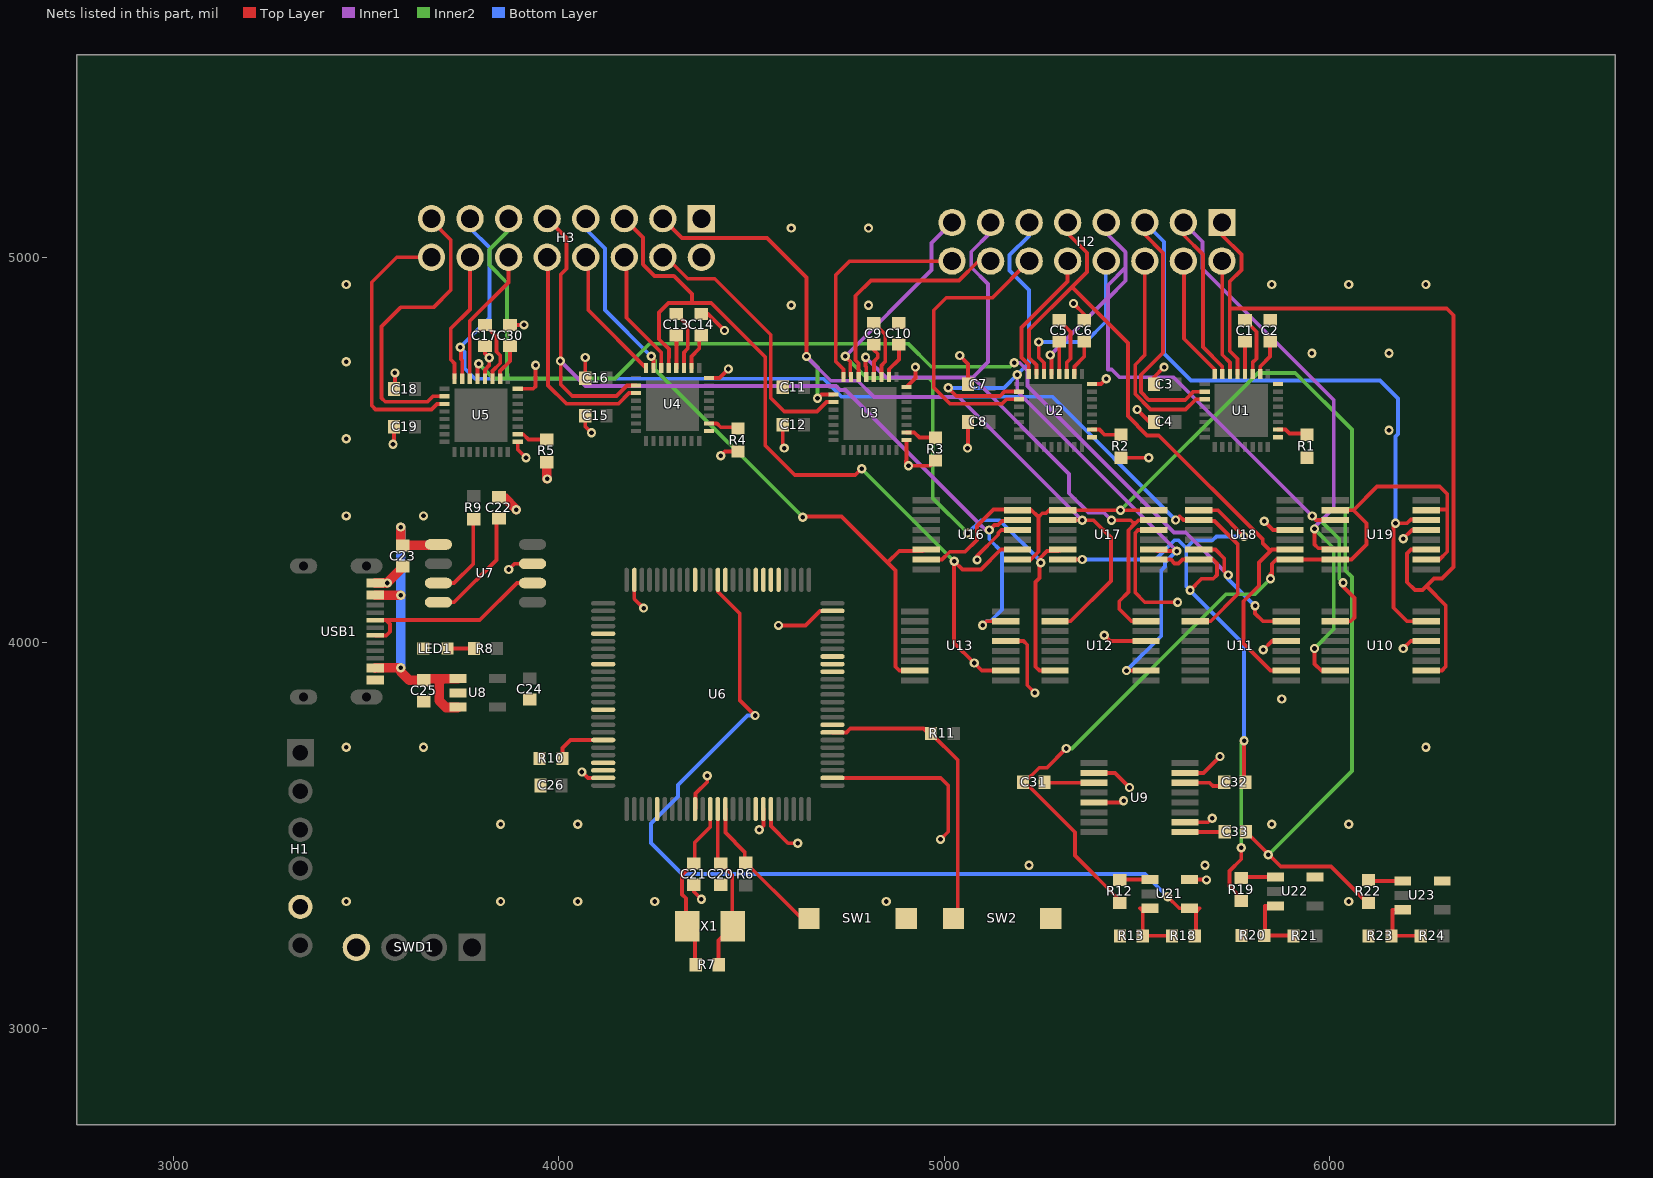
[diagram p0: the nets of this part, all layers, seen from the top]
# Altium PCB MISC49858.pcbdoc (part 2 of 3)
Units mil, origin at the board's own origin, x right, y up, seen from the top; angles counter-clockwise.
Board outline 3990 x 2775 mil, 6 copper layers (Top Layer, Inner1, Inner2, Inner3, Inner4, Bottom Layer), stack 60.565 mil thick; 79 components, 151 nets, 603 pads, 275 vias.

## Via types
v1: diameter 24.02, hole 12, Top Layer to Bottom Layer, 275 vias

## Nets (pads, with @x,y where several pads share a name; then routed paths per layer and width w, separated by ;. In a path a pad name is that pad's centre, name@x,y a point inside that pad or via, vN(x,y) a via of type N, cw(c..) or ccw(c..) an arc to the next point about the centre after c; other vN are vias at no path point) (continued)
$2N132: U7.2 USB1.A7 USB1.B7 | length 550.9
  Top Layer w10: USB1.A7@3524.29,4019.26 3552.56,4019.26 3561.93,4028.63 3561.93,4048.63 3551.93,4058.63 USB1.B7@3524.29,4058.63 3795.2,4058.63 3891.57,4154.99 U7.2@3932,4155
$2N186: C22.1 U7.8 | length 305.9
  Top Layer w10: U7.8@3688,4105 3728.43,4105 3838.43,4214.99 3838.43,4314.99 C22.1@3845,4322.44
$2N192: R9.1 U7.7 | length 227
  Top Layer w10: U7.7@3688,4155 3728.43,4154.99 3778.43,4204.99 3778.43,4314.99 R9.1@3779.66,4320.68
$2N294: LED1.1 R8.1 | length 68.9
  Top Layer w10: LED1.1@3711.47,3985.01 R8.1@3780.34,3985
$2N443: C30.1 U5.26 | length 95.2
  Top Layer w9.92: U5.26@3848.02,4684.78 3848.01,4704.78 3873.59,4730.35 C30.1@3873.59,4769.38
$2N495: R5.2 U5.18 | length 80.8
  Top Layer w9.92: U5.18@3893.59,4540.79 3907.98,4540.79 3921.39,4527.37 R5.2@3968.81,4527.37
$2N1063: C14.1 U4.26 | length 95.2
  Top Layer w9.92: U4.26@4344.43,4712.84 4344.43,4742.84 4364.43,4762.84 4364.43,4791.87 C14.1@4370,4797.44
$2N1115: R4.2 U4.18 | length 80.4
  Top Layer w9.92: U4.18@4390,4568.85 4410,4568.86 4420,4558.86 4460,4558.86 R4.2@4465.22,4555.43
$2N1219: C10.1 U3.26 | length 95.2
  Top Layer w9.92: U3.26@4856.57,4689.46 4856.57,4709.46 4882.14,4735.03 C10.1@4882.14,4774.06
$2N1271: R3.2 U3.18 | length 80.8
  Top Layer w9.92: U3.18@4902.14,4545.47 4922.14,4545.47 4935.56,4532.05 R3.2@4977.36,4532.05
$2N1375: C6.1 U2.26 | length 95.2
  Top Layer w9.92: U2.26@5337.29,4696.84 5337.29,4716.84 5362.87,4742.42 C6.1@5362.87,4781.44
$2N1427: R2.2 U2.18 | length 80.8
  Top Layer w9.92: U2.18@5382.86,4552.85 5402.15,4552.85 5415.57,4539.43 R2.2@5458.08,4539.43
$2N1634: R1.2 U1.18 | length 80.4
  Top Layer w9.92: U1.18@5864.97,4552.85 5884.97,4552.86 5894.97,4542.86 5934.97,4542.86 R1.2@5940.19,4539.43
$2N1686: C2.1 U1.26 | length 95.2
  Top Layer w9.92: U1.26@5819.4,4696.84 5819.4,4716.84 5844.97,4742.42 C2.1@5844.97,4781.44
$2N21184: U6.90
$2N21229: U6.18
$2N21235: U6.34
$2N21247: U6.66
$2N21259: U6.80
$2N21271: U6.84
$2N21286: U6.55
$2N21289: U6.56
$2N21292: U6.57
$2N21295: U6.58
$2N21307: U6.62
$2N21310: U6.97
$2N21317: U6.98
$2N21332: U6.5
$2N21344: U6.41
$2N21348: U6.42
$2N21351: U6.43
$2N24751: R10.1 U6.94 | length 141.3
  Top Layer w10: R10.1@4009.66,3700 4009.66,3726.95 4030.59,3747.88 U6.94@4115.29,3747.88
$2N29551: C32.2 U9.14 | length 109.4
  Top Layer w10: U9.14@5624.33,3636.93 5688.08,3636.93 5696.46,3628.55 5716.46,3628.55 C32.2@5725.93,3638.55
$2N29571: C33.2 U9.9 | length 103.1
  Top Layer w10: U9.9@5624.33,3508.98 5714.83,3508.98 C33.2@5727.44,3510
$2N29592: C31.1 U9.3 | length 129.4
  Top Layer w10: C31.1@5259.37,3638.55 5265.99,3638.55 5267.61,3636.93 U9.3@5388.11,3636.93
$2N29599: R12.2 U21.1 | length 78.6
  Top Layer w10: R12.2@5455,3384.66 5466.88,3386.25 U21.1@5533.53,3386.25
$2N29605: R13.2 R18.1 U21.3 | length 177
  Top Layer w10: U21.3@5533.53,3311.45 5506.88,3311.45 5514.66,3303.67 R13.2@5514.66,3240 R18.1@5590.34,3240
$2N29606: R20.2 R21.1 U22.3 | length 179.7
  Top Layer w10: U22.3@5858.81,3317.6 5832.16,3317.6 5832.16,3247.6 5829.92,3245.36 R20.2@5829.92,3241.02 5899.92,3241.02 R21.1@5905.34,3240
$2N29610: R19.2 U22.1 | length 89.1
  Top Layer w10: R19.2@5770,3389.66 5782.16,3392.4 U22.1@5858.81,3392.4
$2N29613: R23.2 R24.1 U23.3 | length 171
  Top Layer w10: U23.3@6188.81,3307.6 6162.16,3307.6 6162.16,3247.6 6159.66,3245.1 R23.2@6159.66,3240 R24.1@6235.34,3240
$2N29617: R22.2 U23.1 | length 89.8
  Top Layer w10: R22.2@6100,3384.66 6102.16,3382.4 U23.1@6188.81,3382.4
+5V: C23.2 C25.2 U7.5 U8.1 U8.3 USB1.A4B9 USB1.B4A9 | length 927.8
  Top Layer w25: USB1.B4A9@3524.29,3934.61 3524.68,3935 v1(3590,3935) 3590,3925 3612.32,3902.68 C25.2@3650,3902.68 3654.33,3907.01 3700.69,3907.01 ; USB1.A4B9@3524.29,4123.59 v1(3590,4123.59) ; v1(3590,4300) 3590,4257.56 C23.2@3595,4252.56 3685.56,4252.56 U7.5@3688,4255 ; U8.3@3738.82,3832.99 3738.14,3832.32 3707.68,3832.32 3690,3850 3690,3896.32 3700.69,3907.01 ; U8.1@3738.82,3907.01 3700.69,3907.01
  Bottom Layer w25: v1(3590,3935) v1(3590,4123.59) v1(3590,4300)
AC0: C1.2 U1.27 | length 156.2
  Top Layer w9.92: C1.2@5779.97,4836.56 5809.72,4806.84 5809.72,4736.84 5799.72,4726.84 U1.27@5799.72,4696.84
AC1: C1.1 U1.28 | length 84.6
  Top Layer w9.92: C1.1@5779.97,4781.44 5780.03,4776.84 U1.28@5780.03,4696.84
AC2: H2.1 U1.29 U10.2 U19.3 | length 2240.4
  Top Layer w9.92: H2.1@5720,5090 5720.35,5086.84 5720.35,5056.84 5770.35,5006.84 5770.35,4966.84 5740.35,4936.84 5740.35,4866.84 ; U1.29@5760.35,4696.84 5760.35,4736.84 5740.35,4756.84 5740.35,4866.84 ; U19.3@6249.98,4241.53 6240.35,4241.9 6210.35,4241.9 6200.35,4231.9 6200.35,4156.85 6220.35,4136.85 6240.35,4136.85 6270.35,4166.85 6290.35,4166.85 6320.35,4196.85 6320.35,4849.65 6303.16,4866.84 5740.35,4866.84
  Top Layer w10: U10.2@6249.98,3927.83 6260.35,3928.2 6290.35,3928.2 6300.35,3938.2 6300.35,4096.85 6250.35,4146.85
AC3: H2.2 U1.30 | length 301.5
  Top Layer w9.92: H2.2@5720,4990 5720.66,4986.84 5720.66,4746.84 5740.66,4726.84 U1.30@5740.66,4696.84
AC4: H2.3 U1.31 U10.15 U19.14 | length 1963.6
  Top Layer w9.92: H2.3@5620,5090 5620.98,5086.84 5620.98,5056.84 5670.98,5006.84 5670.98,4766.84 5720.98,4716.84 U1.31@5720.98,4696.84 ; v1(5960,4295.3) 5960,4255.3 5970,4245.3 6010,4245.3 U19.14@6013.76,4241.53
  Top Layer w10: v1(5960,3985.3) 5960,3945.3 5977.47,3927.83 U10.15@6013.76,3927.83
  Inner1 w9.92: H2.3@5620,5090 5670,5040 5670,4970 6010,4630 6010,4350 5960,4300 v1(5960,4295.3)
  Inner2 w10: v1(5960,3985.3) 6010,4035.3 6010,4245.3 v1(5960,4295.3)
AC5: H2.4 U1.32 | length 326.5
  Top Layer w9.92: H2.4@5620,4990 5621.29,4986.84 5621.29,4788.71 5701.29,4708.71 U1.32@5701.29,4696.84
AC6: H2.5 U1.2 U10.7 U19.6 | length 2414.6
  Top Layer w9.92: H2.5@5520,5090 5520,5058.63 5567.36,5011.27 5567.36,4752.36 5510,4695 5510,4650 5530,4630 5625,4630 5646.27,4651.27 U1.2@5675.41,4651.27 ; v1(6170,4310) v1@6175,4310 ; 6200,4310 6210,4320 6240,4320 U19.6@6249.98,4318.3
  Top Layer w10: 6200,4310 6175,4310 6165,4300 6165,4090.76 6200,4055.76 U10.7@6249.98,4055.78
  Bottom Layer w9.92: H2.5@5520,5090 5570,5040 5570,4750 5640,4680 6130,4680 6176.38,4633.62 6176.38,4541.5 6170,4535.12 v1(6170,4310)
AC7: H2.6 U1.3 | length 563.3
  Top Layer w9.92: H2.6@5520,4990 5520,4745.93 5495,4720.93 5495,4645 5535,4605 5625.8,4605 5652.4,4631.59 U1.3@5675.41,4631.59
BC0: C5.2 U2.27 | length 156.2
  Top Layer w9.92: C5.2@5297.87,4836.56 5327.61,4806.84 5327.61,4736.84 5317.61,4726.84 U2.27@5317.61,4696.84
BC1: C5.1 U2.28 | length 84.6
  Top Layer w9.92: C5.1@5297.87,4781.44 5297.92,4776.84 U2.28@5297.92,4696.84
BC2: H2.7 U2.29 U10.10 U19.11 | length 1900.9
  Top Layer w9.92: v1(5274.97,4746.5) 5278.24,4743.23 U2.29@5278.24,4696.84
  Top Layer w10: v1(5954.26,4328.8) 5964.26,4318.8 6004.26,4318.8 U19.11@6013.76,4318.3 ; U10.10@6013.76,4055.78 6054.26,4055.78 6064.26,4065.78 6064.26,4115.78 6034.26,4145.78 v1(6034.26,4155.78)
  Inner1 w9.92: v1(5274.97,4746.5) 5421.56,4893.1 5424.26,4893.1 ; H2.7@5420,5090 5420,5063.06 5470,5013.06 5470,4973.06 ; v1(5954.26,4328.8) 5594.26,4688.8 5454.26,4688.8 5434.26,4708.8 5424.26,4708.8 5424.26,4893.1 ; 5424.26,4893.1 5424.26,4927.33 5470,4973.06 ; 5424.26,4893.1 5470,4938.83 5470,4973.06
  Inner2 w10: v1(5954.26,4328.8) 5964.26,4318.8 5974.26,4318.8 6024.26,4268.8 6024.26,4165.78 v1(6034.26,4155.78)
BC3: H2.8 U2.30 | length 441.9
  Top Layer w9.92: v1(5245,4780) 5245,4740 5258.55,4726.45 U2.30@5258.55,4696.84
  Bottom Layer w9.92: v1(5245,4780) 5366.08,4780 5418.55,4832.47 5418.55,4986.84 H2.8@5420,4990
BC4: H2.9 U2.31 U11.2 U18.3 | length 1860.2
  Top Layer w9.92: U2.31@5238.87,4696.84 5238.87,4720.51 5220,4739.39 5220,4811.77 5331.06,4922.83 ; H2.9@5320,5090 5320,5061.76 5370,5011.77 5370,4961.77 5331.06,4922.83 ; 5846.06,4237.83 5826.06,4257.83 5826.06,4267.83 5556.06,4537.83 5526.06,4537.83 5476.06,4587.83 5476.06,4777.83 5331.06,4922.83
  Top Layer w10: U11.2@5886.56,3927.83 5846.06,3927.83 5776.06,3997.83 5776.06,4107.83 5816.06,4147.83 5816.06,4207.83 5846.06,4237.83 5849.77,4241.53 U18.3@5896.56,4241.53
BC5: H2.10 U2.32 | length 350.6
  Top Layer w9.92: U2.32@5219.18,4696.84 5219.18,4720.5 5200,4739.68 5200,4817.66 5319.18,4936.84 5319.18,4986.84 H2.10@5320,4990
BC6: H2.11 U2.2 U12.2 U17.3 | length 1942
  Top Layer w10: v1@5010,4661.1 5031.1,4640 5145,4640 5156.27,4651.27 U2.2@5193.3,4651.27 ; v1(5472.65,3927.83) U12.2@5523.14,3927.83 ; U17.3@5543.14,4241.53 5552.65,4237.83 v1(5602.65,4237.83)
  Inner1 w9.92: v1(5189.2,4695.38) 5189.2,4655.38 5189.2,4651.27 v1(5602.65,4237.83)
  Bottom Layer w9.92: v1(5189.2,4695.38) 5219.2,4725.38 5219.2,4915.38 5169.2,4965.38 5169.2,5005.38 5219.2,5055.38 5219.2,5085.38 H2.11@5220,5090
  Bottom Layer w10: v1@5010,4661.1 5154.93,4661.1 v1(5189.2,4695.38) ; v1(5472.65,3927.83) 5562.65,4017.83 5562.65,4187.83 5572.65,4197.83 5572.65,4207.83 v1(5602.65,4237.83)
  other v1: 5010,4661.25
BC7: H2.12 U2.3 | length 743.5
  Top Layer w9.92: U2.3@5193.3,4631.59 5161.59,4631.59 5150,4620 5015,4620 4972.5,4662.5 4972.5,4862.5 5005,4895 5125,4895 H2.12@5220,4990
C01: C31.2 R12.1 U18.2 U19.2 U19.7 U19.10 U19.15 | length 2296.9
  Top Layer w9.92: v1(5846.06,4165.94) 5850,4169.88 5850,4205 5860.94,4215.94 U18.2@5896.56,4215.94
  Top Layer w10: C31.2@5204.25,3638.55 C31.2@5208.67,3638.55 ; v1(5316.06,3725.94) 5266.06,3675.94 5246.06,3675.94 C31.2@5208.67,3638.55 ; R12.1@5455,3325.34 5455,3332.22 5338.67,3448.55 5338.67,3508.55 C31.2@5208.67,3638.55 ; v1(5846.06,4165.94) 5846.06,4178.94 ; U18.2@5896.56,4215.94 U19.15@6013.76,4215.94 6055.94,4215.94 6095,4255 6095,4310 6061.11,4343.89 ; U19.10@6021.71,4345.94 U19.10@6013.76,4343.89 6061.11,4343.89 ; U19.2@6249.98,4215.94 6284.26,4215.94 6304.26,4235.94 6304.26,4345.94 ; U19.7@6249.98,4343.89 6254.26,4345.94 6304.26,4345.94 ; 6061.11,4343.89 6122.22,4405 6285,4405 6304.26,4385.74 6304.26,4345.94
  Inner2 w10: v1(5316.06,3725.94) 5330.94,3725.94 5730.94,4125.94 5806.06,4125.94 v1(5846.06,4165.94)
C02: C32.1 R19.1 U17.2 U17.15 U18.10 U18.15 | length 2067.2
  Top Layer w10: U17.15@5306.92,4215.94 v1(5357.43,4215.94) ; U17.2@5543.14,4215.94 5587.42,4215.94 5597.42,4205.94 5607.42,4205.94 5617.42,4215.94 5697.42,4215.94 5707.42,4205.94 5707.42,4175.94 5697.42,4165.94 5667.42,4165.94 v1(5637.42,4135.94) ; U18.15@5657.42,4215.94 U18.15@5660.34,4215.94 ; U18.10@5660.34,4343.89 5709.48,4343.89 v1(5777.42,4275.94) ; R19.1@5770,3330.34 5770,3338.52 5740,3368.52 5740,3408.52 5770,3438.52 v1(5770,3468.52) ; v1(5777.42,3745.94) 5777.42,3645.94 C32.1@5781.05,3638.55
  Inner2 w10: v1(5770,3468.52) 5770,3738.52 v1(5777.42,3745.94)
  Bottom Layer w10: v1(5357.43,4215.94) 5547.42,4215.94 5597.42,4265.94 5607.42,4265.94 5627.42,4245.94 ; v1(5777.42,3745.94) 5777.42,3995.94 v1(5637.42,4135.94) 5627.42,4145.94 5627.42,4245.94 ; v1(5777.42,4275.94) 5749.54,4275.94 5749.07,4275.47 5705.47,4275.47 5695.94,4265.94 5647.42,4265.94 5627.42,4245.94
C03: C33.1 R22.1 U16.2 U16.7 U16.15 U17.7 U17.10 | length 3248.1
  Top Layer w10: U16.15@4953.5,4215.94 4994,4215.94 5014,4235.94 5054,4235.94 5085,4266.94 5085,4302.74 5127.72,4345.47 5145.03,4345.47 5145.51,4345.94 U16.7@5194,4345.94 ; U16.2@5189.72,4215.94 5224,4215.94 5244,4235.94 5244,4325.94 ; U16.7@5189.72,4343.89 U16.7@5194,4345.94 ; U17.7@5543.14,4343.89 v1(5457.09,4343.89) U17.10@5306.92,4343.89 5294,4345.94 5274,4345.94 5264,4335.94 5254,4335.94 5244,4325.94 ; C33.1@5782.56,3510 5872.56,3420 6002.56,3420 6097.22,3325.34 R22.1@6100,3325.34 ; U16.7@5194,4345.94 5224,4345.94 5244,4325.94
  Inner2 w10: v1(5457.09,4343.89) 5813.19,4700 5910,4700 6057.25,4552.75 6057.25,4352.22 6040,4334.96 6040,4187.63 6057.25,4170.37 6057.25,3667.25 v1(5840,3450)
CC0: C9.2 U3.27 | length 156.2
  Top Layer w9.92: C9.2@4817.14,4829.18 4846.89,4799.46 4846.89,4729.46 4836.89,4719.46 U3.27@4836.89,4689.46
CC1: C9.1 U3.28 | length 92.8
  Top Layer w9.92: C9.1@4817.14,4774.06 4817.32,4759.34 4827.2,4749.46 4827.2,4739.46 4817.2,4729.46 U3.28@4817.2,4689.46
CC2: H2.13 U3.29 U12.7 U17.6 | length 1788.5
  Top Layer w9.92: v1(4795.79,4740.38) 4795.79,4717.32 4797.52,4715.58 U3.29@4797.52,4689.46 ; v1(5433.65,4317.8) 5483.65,4317.8 5493.65,4307.8
  Top Layer w10: U12.7@5523.14,4055.78 5485.67,4055.78 5453.65,4087.8 5453.65,4107.8 5477.83,4131.99 5477.83,4291.99 5493.65,4307.8 5503.65,4317.8 5533.65,4317.8 U17.6@5543.14,4318.3
  Inner1 w9.92: v1(4795.79,4740.38) 4848.37,4687.8 5073.65,4687.8 ; H2.13@5120,5090 5120,5064.15 5070,5014.15 5070,4974.15 5113.65,4930.51 5113.65,4727.8 5073.65,4687.8 ; v1(5433.65,4317.8) 5413.65,4337.8 5373.65,4337.8 5323.65,4387.8 5323.65,4437.8 5073.65,4687.8
CC3: H2.14 U3.30 | length 600.9
  Top Layer w9.92: U3.30@4777.83,4689.46 4777.83,4725 4770,4732.83 4770,4900 4809.46,4939.46 5037.83,4939.46 5087.83,4989.46 5107.83,4989.46 H2.14@5120,4990
CC4: H2.15 U3.31 U12.15 U17.14 | length 1881
  Top Layer w9.92: v1@5246.43,4207.83 v1@5253.21,4207.83
  Top Layer w10: v1(4742.93,4742.83) 4756.02,4729.74 4756.02,4691.59 U3.31@4758.15,4689.46 ; v1@5253.21,4207.83 5249.86,4204.48 v1@5246.43,4204.48 ; U12.15@5286.92,3927.83 5246.43,3927.83 5236.43,3937.83 5236.43,4157.83 5246.43,4167.83 v1@5246.43,4204.48 ; U17.14@5306.92,4241.53 5296.43,4237.83 5266.43,4237.83 5246.43,4217.83 5246.43,4207.83 v1@5246.43,4204.48
  Inner1 w9.92: v1(4742.93,4742.83) 4966.52,4966.42 4966.52,5036.52 H2.15@5020,5090
  Inner2 w9.92: v1(4742.93,4742.83) 4798.92,4686.84 4959.86,4686.84 4969.78,4676.92 4969.78,4375.49 v1(5060.91,4284.36)
  Bottom Layer w9.92: v1(5060.91,4284.36) 5094.38,4317.83 5143.21,4317.83 v1@5253.21,4207.83
  other v1: 5249.78,4207.83
CC5: H2.16 U3.32 | length 588.8
  Top Layer w9.92: U3.32@4738.46,4689.46 4738.46,4709.46 4718.46,4729.46 4718.46,4953.46 4754.46,4989.46 5008.46,4989.46 H2.16@5020,4990
CC6: H3.3 U3.2 U12.10 U17.11 | length 2142.3
  Top Layer w9.92: H3.3@4270,5100 4320,5050 4540,5050 4642.43,4947.57 v1(4642.43,4742.8) ; v1(4671.11,4633.89) 4681.11,4643.89 U3.2@4712.58,4643.89
  Top Layer w10: U12.10@5286.92,4055.78 5327.43,4055.78 5431.85,4160.2 5431.85,4273.15 5387.2,4317.8 v1(5357.43,4317.8) 5317.43,4317.8 U17.11@5306.92,4318.3
  Inner1 w9.92: v1(4642.43,4742.8) 4705.51,4679.71 4775.51,4679.71 4817.43,4637.8 5037.43,4637.8 v1(5357.43,4317.8)
  Inner2 w9.92: v1(4642.43,4742.8) 4671.11,4714.12 v1(4671.11,4633.89)
CC7: H3.4 U3.3 | length 714.2
  Top Layer w9.92: H3.4@4270,5000 4278.74,5000 4334.53,4944.21 4404.53,4944.21 4550,4798.74 4550,4635 4585,4600 4670,4600 4694.21,4624.21 U3.3@4712.58,4624.21
DC0: C13.2 U4.27 | length 156.2
  Top Layer w9.92: C13.2@4305,4852.56 4334.75,4822.84 4334.75,4762.84 4324.75,4752.84 U4.27@4324.75,4712.84
DC1: C13.1 U4.28 | length 84.6
  Top Layer w9.92: C13.1@4305,4797.44 U4.28@4305.06,4712.84
DC2: H3.5 U4.29 U13.2 U16.3 | length 2246.9
  Top Layer w9.92: H3.5@4170,5100 4218.47,5051.53 4218.47,4981.53 4248.47,4951.53 4298.47,4951.53 4345.52,4904.48 4345.52,4881.53 ; U4.29@4285.38,4712.84 4285.52,4761.53 4260,4787.05 4260,4856.5 4285.03,4881.53 4345.52,4881.53 ; v1(4785.52,4451.53) 4768.99,4435 4612.05,4435 4535.52,4511.53 4535.52,4741.53 4395.52,4881.53 4345.52,4881.53 ; U13.2@5159.72,3927.83 5097.17,3927.83 v1(5077.48,3947.52) 5025.52,3999.48 v1(5025.52,4211.53) 5047.05,4190 5095,4190 5146.53,4241.53 U16.3@5189.72,4241.53
  Inner2 w9.92: v1(4785.52,4451.53) v1(5025.52,4211.53)
DC3: H3.6 U4.30 | length 326.4
  Top Layer w9.92: H3.6@4170,5000 4175.69,4992.84 4175.69,4842.84 4265.69,4752.84 U4.30@4265.69,4712.84
DC4: H3.7 U4.31 U13.15 U16.14 | length 1768.2
  Top Layer w9.92: v1(4240,4742.84) 4246.01,4736.84 U4.31@4246.01,4712.84 ; v1(4633.01,4325.85) 4633.01,4317.83 4643.01,4327.83 4733.01,4327.83 4853,4207.83
  Top Layer w10: U13.15@4923.5,3927.83 4883,3927.83 4873,3937.83 4873,4187.83 4853,4207.83 4883,4237.83 4943,4237.83 U16.14@4953.5,4241.53
  Inner2 w9.92: v1(4240,4742.84) 4250,4732.84 4250,4708.85 v1(4633.01,4325.85)
  Bottom Layer w9.92: H3.7@4070,5100 4070,5072.84 4120,5022.84 4120,4862.84 v1(4240,4742.84)
DC5: H3.8 U4.32 | length 351.7
  Top Layer w9.92: H3.8@4070,5000 4076.32,4992.84 4076.32,4862.84 U4.32@4226.32,4712.84
DC6: H3.9 U4.2 U13.7 U16.6 | length 2405.3
  Top Layer w9.92: H3.9@3970,5100 4020,5050 4020,4970 4005,4955 4005,4670 4035,4640 4150,4640 4177.27,4667.27 U4.2@4200.44,4667.27
  Top Layer w10: v1(5099.22,4045.78) 5109.22,4055.78 U13.7@5159.72,4055.78 ; v1(5116.47,4292.42) 5129.83,4305.78 5139.22,4305.78 5149.22,4315.78 5187.2,4315.78 U16.6@5189.72,4318.3
  Inner1 w9.92: v1(4004.23,4730.78) 4069.23,4665.78 4719.23,4665.78 4729.23,4655.78 4743.26,4655.78 5106.61,4292.42 v1(5116.47,4292.42)
  Bottom Layer w10: v1(5099.22,4045.78) 5109.22,4055.78 5119.22,4055.78 5149.22,4085.78 5149.22,4235.78 5116.47,4268.53 v1(5116.47,4292.42)
DC7: H3.10 U4.3 | length 591.8
  Top Layer w9.92: H3.10@3970,5000 3972.39,4987.6 3972.39,4667.61 4020,4620 4155,4620 4182.59,4647.59 U4.3@4200.44,4647.59
EC0: C17.2 U5.27 | length 164.5
  Top Layer w9.92: C17.2@3808.59,4824.5 3838.34,4794.78 3838.34,4754.78 3848.34,4744.78 3848.34,4724.81 3828.34,4704.81 U5.27@3828.34,4684.78
EC1: C17.1 U5.28 | length 93.6
  Top Layer w9.92: C17.1@3808.59,4769.38 3808.59,4750.03 v1(3819.52,4739.1) 3819.52,4718.71 3808.65,4707.83 U5.28@3808.65,4684.78
EC2: H3.11 U5.29 U11.7 U18.14 | length 3112.1
  Top Layer w9.92: U5.29@3788.97,4684.78 3788.97,4720.61 v1(3792.27,4723.92)
  Top Layer w10: U18.14@5660.34,4241.53 5703.47,4241.53 5726.06,4218.94 5726.06,4185.78 v1(5736.06,4175.78) ; v1(5806.06,4095.78) 5806.06,4075.78 5826.06,4055.78 U11.7@5886.56,4055.78
  Inner1 w9.92: v1(5181.06,4726.15) 5195.69,4726.15 5216.06,4705.78 5216.06,4665.78 5596.06,4285.78 5626.06,4285.78 v1(5736.06,4175.78)
  Inner2 w9.92: v1(3792.27,4723.92) 3830.42,4685.78 3866.07,4685.78 ; H3.11@3870,5100 3870,5069.71 3820,5019.71 3820,4979.71 3866.07,4933.64 3866.07,4685.78 ; v1(5181.06,4726.15) 5170.69,4715.78 4966.06,4715.78 4906.06,4775.78 4236.07,4775.78 4146.07,4685.78 3866.07,4685.78
  Bottom Layer w10: v1(5736.06,4175.78) 5736.06,4165.78 v1(5806.06,4095.78)
EC3: H3.12 U5.30 | length 356.7
  Top Layer w9.92: U5.30@3769.28,4684.78 3769.28,4834.78 3869.27,4934.78 3869.27,4994.78 H3.12@3870,5000
EC4: H3.13 U5.31 U11.10 U18.11 | length 3000.6
  Top Layer w9.92: v1(3744.22,4766.54) 3746.36,4764.4 3746.36,4735.85 3749.6,4732.62 U5.31@3749.6,4684.78 ; v1(5599.88,4318.3) 5609.88,4328.3 5619.88,4318.3 U18.11@5660.34,4318.3
  Top Layer w10: U11.10@5650.34,4055.78 5690.84,4055.78 5760.84,4125.78 5760.84,4255.78 5700.84,4315.78 5662.87,4315.78 U18.11@5660.34,4318.3
  Bottom Layer w9.92: H3.13@3770,5100 3770,5075.18 3820,5025.18 3820,4842.32 v1(3744.22,4766.54) 3756.36,4754.4 3756.36,4711.54 3783.12,4684.78 4686.36,4684.78 4732.84,4638.3 5279.88,4638.3 v1(5599.88,4318.3)
EC5: H3.14 U5.32 | length 340.1
  Top Layer w9.92: U5.32@3729.91,4684.78 3729.9,4724.78 3719.9,4734.78 3719.9,4814.78 3769.9,4864.78 3769.9,4994.78 H3.14@3770,5000
EC6: H3.15 U5.2 | length 784.1
  Top Layer w9.92: H3.15@3670,5100 3670,5095 3720,5045 3720,4915 3675,4870 3590,4870 3540,4820 3540,4635 3550,4625 3660,4625 3674.21,4639.21 U5.2@3704.03,4639.21
EC7: H3.16 U5.3 | length 701.1
  Top Layer w9.92: H3.16@3670,5000 3580,5000 3515,4935 3515,4615 3525,4605 3670,4605 3684.53,4619.53 U5.3@3704.03,4619.53
GND: C2.2 C3.1 C4.1 C6.2 C7.1 C8.1 C10.2 C11.1 C12.1 C14.2 C15.1 C16.1 C18.1 C19.1 C20.1 C21.1 C22.2 C23.1 C24.1 C25.1 C26.1 C30.2 H1.5 H3.1 H3.2 LED1.2 R1.1 R2.1 R3.1 R4.1 R5.1 R10.2 R13.1 R20.1 R23.1 SW1.1 SW2.1 SWD1.4 U1.17 U1.24 U2.17 U2.24 U3.17 U3.24 U4.17 U4.24 U5.17 U5.24 U6.10 U6.19 U6.20 U6.27 U6.49 U6.74 U6.99 U7.3 U8.2 U9.2 U9.5 U9.10 U9.15 U10.5 U11.5 U12.5 U13.5 U16.5 U17.5 U18.5 U19.5 U21.5 U22.5 U23.5 USB1.A1B12 USB1.B1A12 | length 4102.8
  Top Layer w9.92: v1(3570,4515) 3572.44,4517.44 C19.1@3572.44,4560.61 ; C18.1@3572.44,4658.05 3575,4660.61 v1(3575,4700) ; v1(3870,4190) 3885,4205 U7.3@3932,4205 ; C30.2@3873.59,4824.5 v1(3910,4824.5) ; U5.17@3893.59,4521.1 3893.59,4501.41 v1(3915,4480) ; U5.24@3893.59,4658.9 3933.9,4658.9 3940,4665 v1(3940,4720) ; v1(4060,3665) 4075.55,3649.45 U6.99@4115.29,3649.45 ; C15.1@4068.85,4588.67 4068.85,4561.15 v1(4085,4545) ; C16.1@4068.85,4686.11 v1(4068.85,4740) ; U6.74@4195.99,4163.23 4195.99,4114.01 v1(4220,4090) ; C21.1@4350,3372.44 4350,3355 v1(4370,3335) ; U6.10@4353.47,3568.75 4355,3570.27 4355,3608.71 4385,3638.71 v1(4385,3655) ; C14.2@4370,4852.56 4387.44,4852.56 v1(4430,4810) ; U4.24@4390,4686.96 4416.96,4686.96 v1(4440,4710) ; v1(4420,4485) 4431.11,4496.11 R4.1@4465.22,4496.11 ; v1(4520,3515) 4530.64,3525.64 U6.19@4530.64,3568.75 ; U6.20@4550.33,3568.75 4550.33,3524.67 4595,3480 v1(4620,3480) ; v1(4570,4045) 4640,4045 4677.53,4082.53 U6.49@4709.77,4082.53 ; C12.1@4580.99,4565.29 4580.99,4509.01 v1(4585,4505) ; U6.27@4709.77,3649.45 4990.55,3649.45 5010,3630 5010,3510 v1(4990,3490) ; U3.17@4902.14,4525.78 4902.14,4474.28 4900,4472.14 4900,4466.57 v1(4907.22,4459.36) 4963.99,4459.36 R3.1@4977.36,4472.73 ; U3.24@4902.14,4663.58 4925,4686.44 v1(4925,4715) ; v1(5040,4745) 5061.71,4723.29 C7.1@5061.71,4670.11 ; v1(5060,4505) 5061.72,4506.72 C8.1@5061.72,4572.67 ; v1(5085,4215) 5085,4225 5140,4280 5140,4285 5147.71,4292.71 U16.5@5189.72,4292.71 ; U13.5@5159.72,4004.6 5205.4,4004.6 5215,3995 5215,3890 v1(5235,3870) ; v1(5335,4880) 5362.87,4852.13 C6.2@5362.87,4836.56 ; U2.24@5382.86,4670.96 5405.96,4670.96 v1(5420,4685) ; U9.5@5388.11,3585.75 5460.75,3585.75 v1(5465,3590) ; U9.2@5388.11,3662.52 5442.48,3662.52 v1(5480.26,3624.74) ; v1(5415,4019.85) 5430.25,4004.6 U12.5@5523.14,4004.6 ; R2.1@5458.08,4480.11 v1(5530,4480.11) ; v1(5500,4605) 5532.33,4572.67 C4.1@5543.82,4572.67 ; U17.5@5543.14,4292.71 5502.71,4292.71 5495,4285 5495,4130 5520,4105 v1(5605,4105) ; C3.1@5543.82,4670.11 5543.82,4688.82 v1(5570,4715) ; U9.10@5624.33,3534.57 5684.57,3534.57 v1(5695,3545) ; U9.15@5624.33,3662.52 5672.52,3662.52 v1(5715,3705) ; U21.5@5635.9,3386.25 5678.75,3386.25 v1(5680,3385) ; v1(5827.34,3981.91) 5850.04,4004.6 U11.5@5886.56,4004.6 ; v1(5830,4315) 5852.29,4292.71 U18.5@5896.56,4292.71 ; v1(6190,3985) 6209.6,4004.6 U10.5@6249.98,4004.6 ; v1(6190,4270) 6212.71,4292.71 U19.5@6249.98,4292.71
  Top Layer w25: USB1.A1B12@3524.29,4155.09 v1(3555,4155.09) 3595,4195.08 C23.1@3595,4197.44 ; C22.2@3845,4377.56 3857.44,4377.56 v1(3890,4345) ; R5.1@3968.81,4468.05 3968.81,4426.19 v1(3970,4425)
  other v1: 3449.1,3329.1 3849.1,3329.1 4049.1,3329.1 4249.1,3329.1 4849.1,3329.1 6049.1,3329.1 5219.75,3423.22 5676.19,3423.22 3849.1,3529.1 4049.1,3529.1 5849.1,3529.1 6049.1,3529.1 3449.1,3729.1 3649.1,3729.1 6249.1,3729.1 5874.9,3854.27 3449.1,4329.1 3649.1,4329.1 3449.1,4529.1 6153.43,4551.01 3449.1,4729.1 5953.43,4751.01 6153.43,4751.01 4603.23,4875.52 4803.23,4875.52 3449.1,4929.1 5849.1,4929.1 6049.1,4929.1 6249.1,4929.1 4603.23,5075.52 4803.23,5075.52
K1: R11.1 SW2.2 U6.33 | length 778.3
  Top Layer w10: U6.33@4709.77,3767.56 4746.18,3767.56 4756.18,3777.56 4946.18,3777.56 4958.74,3765 R11.1@4965.34,3765 5035,3695.34 5035,3295.99 SW2.2@5024.01,3285
NRST1: R6.1 SW1.2 U6.14 | length 385.1
  Top Layer w10: U6.14@4432.22,3568.75 4432.22,3507.78 4482.22,3457.78 4482.22,3432.34 R6.1@4485,3429.66 4625,3289.66 4645,3289.66 SW1.2@4649.01,3285
OSC_IN: C21.2 R7.2 U6.12 X1.2 | length 447.7
  Top Layer w10: R7.2@4355.34,3165 4353.11,3175 4353.11,3245 X1.2@4333.11,3265 4330,3267.56 4330,3337.56 4320,3347.56 4320,3397.56 C21.2@4350,3427.56 4352.85,3432.34 4352.85,3482.34 4392.85,3522.34 U6.12@4392.85,3568.75
OSC_OUT: C20.2 R7.1 U6.13 X1.1 | length 434.7
  Top Layer w10: U6.13@4412.53,3568.75 4412.53,3435.03 C20.2@4420,3427.56 4450,3397.56 4450,3267.56 X1.1@4451.22,3265 4414.66,3228.45 R7.1@4414.66,3165
OUT1: R18.2 U6.63 U21.4 | length 2416.3
  Top Layer w10: U6.63@4412.53,4163.23 4412.53,4133.23 4469.25,4076.51 4469.25,3851.45 v1(4509.25,3811.45) ; v1(5579.25,3341.45) 5609.25,3311.45 5635.9,3311.45 5662.56,3311.45 5652.56,3301.45 5652.56,3242.9 R18.2@5649.66,3240
  Bottom Layer w10: v1(4509.25,3811.45) 4489.25,3811.45 4309.25,3631.45 4309.25,3601.45 4239.25,3531.45 4239.25,3480.75 4320,3400 5520.7,3400 v1(5579.25,3341.45)